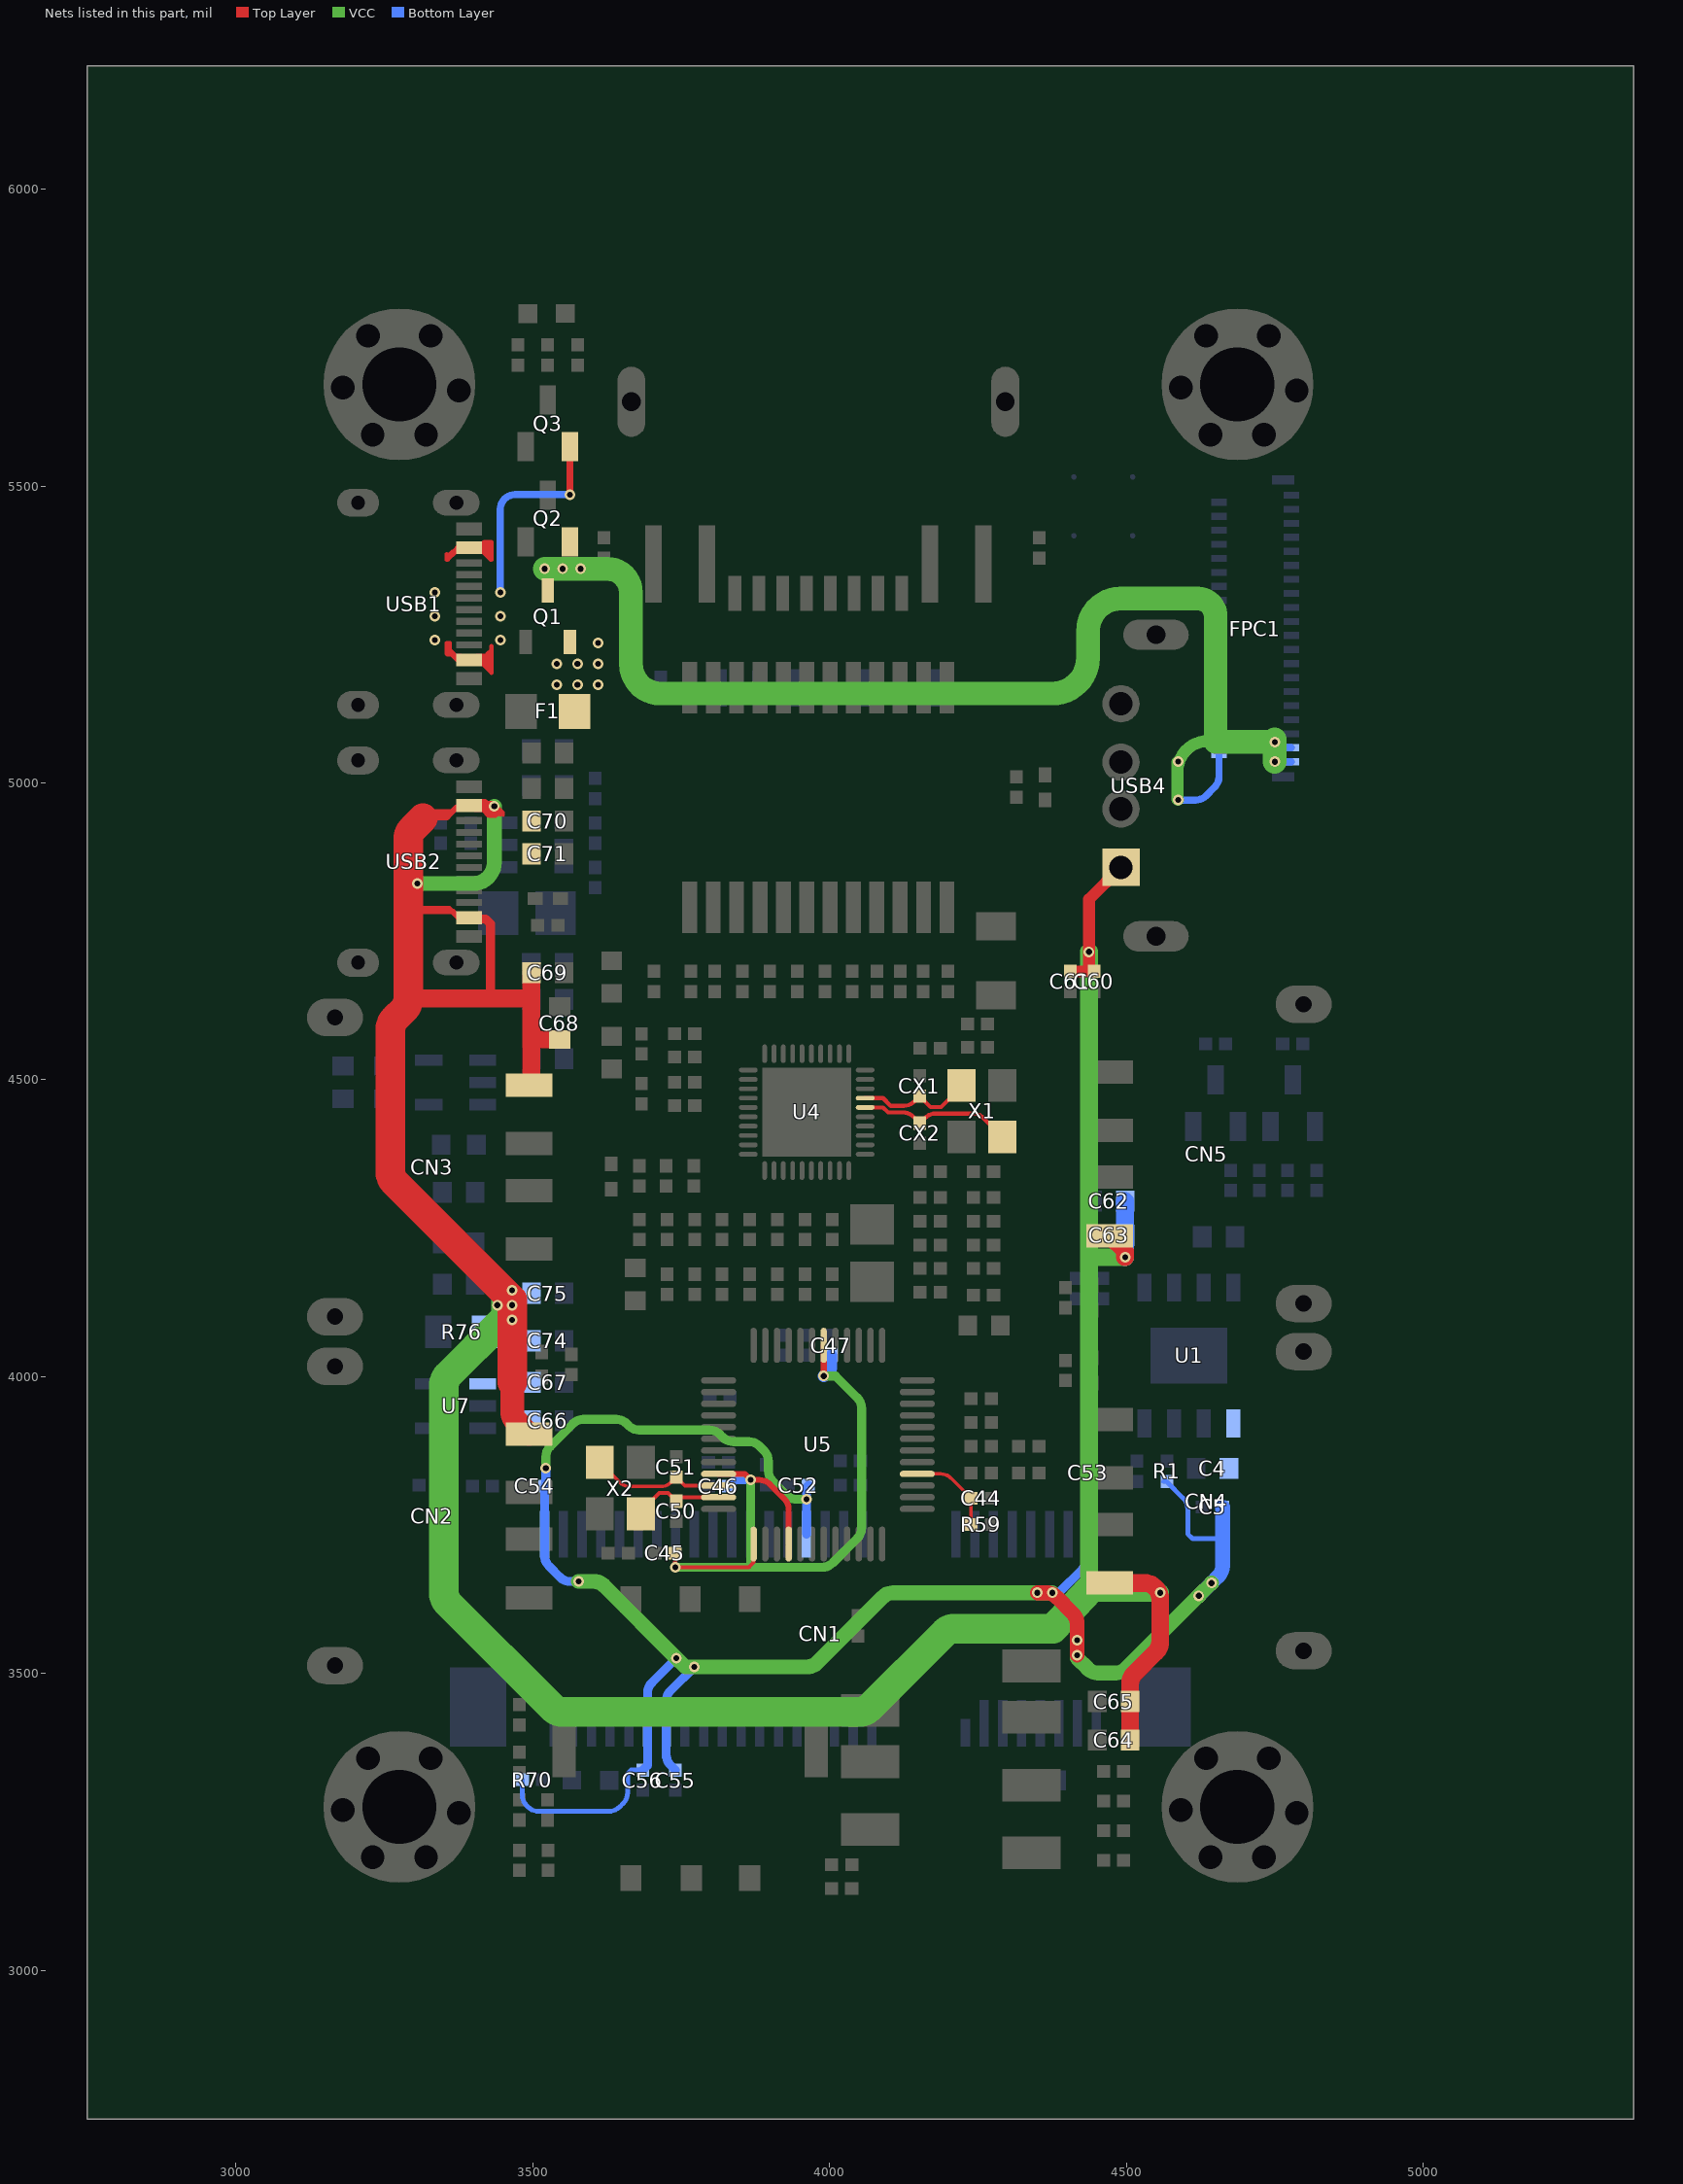
[diagram p0: the nets of this part, all layers, seen from the top]
# Altium PCB MISC84334.PcbDoc (part 8 of 8)
Units mil, origin at the board's own origin, x right, y up, seen from the top; angles counter-clockwise.
Board outline 2605.13 x 3457.4 mil, 4 copper layers (Top Layer, GND, VCC, Bottom Layer), stack 62.447 mil thick; 209 components, 149 nets, 735 pads, 529 vias.

## Via types
v1: diameter 18, hole 10, Top Layer to Bottom Layer, 529 vias

## Nets (pads, with @x,y where several pads share a name; then routed paths per layer and width w, separated by ;. In a path a pad name is that pad's centre, name@x,y a point inside that pad or via, vN(x,y) a via of type N, cw(c..) or ccw(c..) an arc to the next point about the centre after c; other vN are vias at no path point) (continued)
VCC5V0_SYS: FPC1.1 FPC1.2 FPC1.3 FPC1.4 Q1.3 Q2.2 | length 2196
  VCC w20: v1(4587.29,4971.19) 4586.29,4972.19 4586.29,5019.08 ; v1(4587.29,5036.19) 4586.29,5035.19 4586.29,5019.08 ; 4640.59,5070.59 4637.8,5070.59 ccw(c4637.8,5019.08) 4589.01,5035.61 ccw(c4637.8,5019.08) 4586.29,5019.08
  VCC w40: v1(3520.59,5360.59) v1(3550.59,5360.59) v1(3580.59,5360.59) 3625.59,5360.59 cw(c3625.59,5320.59) 3665.59,5320.59 3665.59,5200.59 ccw(c3715.59,5200.59) 3715.59,5150.59 4375.59,5150.59 ccw(c4375.59,5210.59) 4435.59,5210.59 4435.59,5255.59 cw(c4490.59,5255.59) 4490.59,5310.59 4620.59,5310.59 cw(c4620.59,5280.59) 4650.59,5280.59 4650.59,5069.06 v1(4750.2,5069.06) ; v1(4750.29,5035.68) 4750.29,5069.06 v1@4750.29,5073.19
  Bottom Layer w12: v1(4587.29,4971.19) 4616.94,4971.19 ccw(c4616.94,4996.19) 4634.61,4978.51 4648.95,4992.85 ccw(c4631.27,5010.53) 4656.27,5010.53 FPC1.2@4656.27,5047.49 ; v1(4587.29,5036.19) 4614.89,5063.79 cw(c4632.57,5046.11) 4632.57,5071.11 FPC1.4@4656.27,5071.11 ; v1(4750.2,5069.06) 4759.95,5059.3 FPC1.3@4778.31,5059.3 ; v1(4750.29,5035.68) FPC1.1@4778.31,5035.68
VCC5V0_USB_HOST: C60.2 C61.2 C62.2 C63.2 C64.2 C65.2 C66.2 C67.2 C68.2 C69.2 C70.2 C71.2 C74.2 C75.2 CN2.1 CN3.1 CN4.1 CN5.1 R76.2 U7.1 USB2.2 USB2.11 USB4.1 | length 6504.3
  Top Layer w5: 3310.59,4781.94 3363.71,4781.94 USB2.11@3374.22,4771.43 ; 3313.18,4785.39 3313.32,4785.53 3365.65,4785.53 ; 3313.47,4787.58 3357.58,4787.58 3360.59,4790.59 ; 3315.59,4790.59 3360.59,4790.59 ; USB2.11@3388.24,4777.74 3374.8,4777.74 3367.01,4785.53 3365.65,4785.53 ; USB2.2@3402.68,4953.54 3415.71,4953.54 3426.01,4943.23 3437.26,4943.23 3437.72,4943.7 ; USB2.2@3408.37,4965.07 3415.8,4965.07 ; USB2.2@3410.86,4970.27 3420.68,4970.27 3428.42,4962.53 v1@3437.53,4962.53 ; USB2.2@3412.04,4966.85 3419.47,4966.85 3427.01,4959.32 3439.46,4959.32 3445.59,4953.18 3445.59,4945.59 ; 3414.96,4954.56 3414.96,4959.32 ; 3425.84,4967.44 3433.93,4967.44 v1@3438.83,4962.53 ; v1(3435.59,4960.59) v1@3437.53,4962.53 ; 3437.77,4947.77 3426.51,4947.77 3423.04,4951.24 ; 3438.76,4951.24 3423.04,4951.24 ; 3440.59,4945.59 3440.59,4953.67 3438.81,4955.45 3425.42,4955.45 3415.8,4965.07 ; 3450.59,4945.59 3450.59,4950.77 v1@3438.83,4962.53 ; 3360.59,4790.59 3365.65,4785.53 ; 3414.96,4959.32 3423.04,4951.24 ; 3414.96,4959.32 3414.96,4964.23 3415.8,4965.07 ; v1@3437.53,4962.53 v1@3438.83,4962.53
  Top Layer w7: 3331.16,4950.71 3332.7,4952.25 3362.98,4952.25 3371.57,4960.84 3391.86,4960.84 USB2.2@3393.1,4962.08 ; 3333.25,4944.35 3352.35,4944.35 3356.11,4940.59 ; 3334.31,4948.02 3361.5,4948.02 3362.52,4947 ; 3335.59,4940.59 3356.11,4940.59 ; USB2.2@3385.82,4955.77 3371.29,4955.77 3362.52,4947 ; 3356.11,4940.59 3362.52,4947
  Top Layer w15: USB2.11@3391.15,4771.09 3420.52,4771.09 3428.97,4762.64 3428.97,4639.72 3429.51,4639.18
  Top Layer w20: C61.2@4405.59,4682.63 4432.75,4682.63 ; C60.2@4445.59,4682.63 4432.75,4682.63 ; USB4.1@4491.06,4857.8 4437.29,4804.03 v1(4437.29,4715.59) 4437.29,4687.17 4432.75,4682.63
  Top Layer w30: 3300.59,4630.59 3307.01,4637.01 3498.03,4637.01 ; CN3.1@3493.98,4490.89 3498.03,4494.94 3498.03,4567.79 ; C69.2@3498.03,4680.59 3498.03,4637.01 ; 3498.27,4568.03 3498.03,4567.79 ; 3505.59,4568.03 C68.2@3545.59,4568.03 ; CN4.1@4472.2,3652.58 4530.55,3652.58 cw(c4530.55,3627.58) 4548.22,3645.26 4549.97,3643.51 cw(c4532.29,3625.84) 4555.39,3635.4 cw(c4532.29,3625.84) 4557.29,3625.84 4557.29,3554.05 cw(c4532.29,3554.05) 4549.97,3536.37 4513.84,3500.24 ccw(c4531.52,3482.56) 4506.52,3482.56 C65.2@4506.52,3453.09 C64.2@4506.52,3388.09 ; CN5.1@4472.2,4237.58 4498.15,4211.63 v1(4498.15,4201.19) ; 3498.03,4567.79 3498.03,4637.01
  Top Layer w40: 3465.59,3990.59 3465.59,3942.14 ccw(c3490.59,3942.14) 3472.91,3924.46 CN2.1@3493.98,3903.39
  Top Layer w50: 3315.59,4940.59 3297.91,4922.91 ccw(c3315.59,4905.24) 3290.59,4905.24 3290.59,4635.95 cw(c3265.59,4635.95) 3283.27,4618.27 3267.91,4602.91 ccw(c3285.59,4585.24) 3260.59,4585.24 3260.59,4344.95 ccw(c3285.59,4344.95) 3267.91,4327.27 3465.59,4129.59 v1(3465.59,4120.59) v1(3465.59,4095.59) 3465.59,3990.59
  VCC w25: v1(3305.59,4830.59) 3399.78,4830.59 ccw(c3399.78,4866.4) 3435.59,4866.4 v1(3435.59,4960.59)
  VCC w30: v1(4437.29,4715.59) 4437.29,4199.3 ; v1(4498.15,4201.19) 4439.18,4201.19 4437.29,4199.3 ; v1(4557.29,3636.19) 4456.86,3636.19 ; 4437.29,3655.76 4437.29,3640.92 4437.29,3631.19 4442.29,3636.19 4456.86,3636.19 ; 4437.29,3655.76 4437.29,4199.3 ; 4437.29,3655.76 4456.86,3636.19
  VCC w50: 3455.59,4135.59 3455.59,4110.95 cw(c3430.59,4110.95) 3453.48,4100.9 cw(c3430.59,4110.95) 3448.27,4093.27 3357.91,4002.91 ccw(c3375.59,3985.24) 3350.59,3985.24 3350.59,3635.95 ccw(c3375.59,3635.95) 3357.91,3618.27 3533.27,3442.91 ccw(c3550.95,3460.59) 3550.95,3435.59 4050.24,3435.59 ccw(c4050.24,3460.59) 4067.91,3442.91 4193.27,3568.27 cw(c4210.95,3550.59) 4210.95,3575.59 4376.54,3575.59 4378.16,3577.21 ccw(c4360.48,3594.88) 4378.81,3577.88 4437.29,3640.92
  Bottom Layer w30: v1(4498.15,4201.19) C63.2@4498.15,4238.09 C62.2@4498.15,4295.59
  other v1: 3440.59,4120.59 3465.59,4145.59
VCC5V0_USB_VBUS: F1.1 Q1.2 Q3.2 USB1.2 USB1.11 | length 891.9
  Top Layer w7: 3355.59,5385.59 3355.59,5380.59 ; 3359.37,5221.75 3359.37,5219.4 3356.45,5216.48 ; USB1.2@3373.17,5395.16 3370.55,5392.54 3370.55,5389.77 ; USB1.11@3373.2,5206.78 3363.49,5216.48 3356.45,5216.48 ; USB1.2@3375.95,5399.08 3366.64,5389.77 ; USB1.2@3376.74,5389.28 3370.55,5389.28 ; USB1.11@3378.12,5214.41 3370.34,5214.41 3360.59,5224.16 3360.59,5235.59 3355.59,5235.59 3355.59,5217.34 3356.45,5216.48 ; USB1.11@3393.1,5207.1 3409.09,5207.1 3430.59,5185.59 3430.59,5223.59 ; USB1.2@3401.43,5391.03 3413.85,5391.03 3429.29,5375.59 3430.59,5375.59 3430.59,5405.59 ; USB1.11@3406.81,5214.49 3414.83,5214.49 ; USB1.11@3414.18,5203.92 3414.83,5204.56 3414.83,5214.49 ; 3417.14,5390.24 3418.19,5391.29 3418.19,5405.59 ; 3418,5202.33 3418,5211 3421.49,5214.49 ; 3421.4,5388.01 3421.4,5402.38 3418.19,5405.59 ; 3421.78,5197.22 3421.78,5214.2 3421.49,5214.49 ; 3425.92,5193.17 3425.92,5217.22 3425.07,5218.07 ; 3426.1,5381.16 3426.1,5401.1 3430.59,5405.59 ; 3430.59,5230.59 3430.59,5223.59 ; 3355.59,5380.59 3364.77,5389.77 3366.64,5389.77 ; 3355.59,5380.59 3355.59,5375.59 3356.86,5375.59 3370.55,5389.28 ; 3366.64,5389.77 3370.55,5389.77 ; 3370.55,5389.28 3370.55,5389.77 ; 3370.55,5389.77 3386.79,5389.77 USB1.2@3393.1,5396.08 3408.68,5396.08 3418.19,5405.59 ; 3414.83,5214.49 3421.49,5214.49 ; 3418.19,5405.59 3430.59,5405.59 ; 3421.49,5214.49 3425.07,5218.07 ; 3425.07,5218.07 3430.59,5223.59
  Top Layer w12: v1(3562.99,5485.59) Q3.2@3562.99,5566.22
  Bottom Layer w12: v1(3445.59,5320.59) 3445.59,5460.59 cw(c3470.59,5460.59) 3470.59,5485.59 v1(3562.99,5485.59)
  other v1: 3540.59,5165.59 3575.59,5165.59 3610.59,5165.59 3540.59,5200.59 3575.59,5200.59 3610.59,5200.59 3610.59,5235.59 3335.59,5240.59 3445.59,5240.59 3335.59,5280.59 3445.59,5280.59 3335.59,5320.59
VCC_1V8_USB: C45.2 C46.2 C47.2 U5.6 U5.21 U5.25 U5.28 | length 1314.8
  Top Layer w7: C45.2@3740.18,3703.09 v1(3740.18,3679.19) 3864.29,3679.19 3872.32,3687.22 U5.25@3872.32,3718.27
  Top Layer w10: U5.21@3813.27,3836.38 3857.1,3836.38 v1(3867.29,3826.19) 3881.94,3826.19 cw(c3881.94,3801.19) 3899.61,3818.87 3924.06,3794.42 cw(c3906.38,3776.75) 3931.38,3776.75 U5.28@3931.38,3718.27 ; v1(3990.43,4001.19) U5.6@3990.43,4052.91
  VCC w15: v1(3740.18,3679.19) 3868.74,3679.19 ; v1(3867.29,3826.19) 3867.29,3680.64 3868.74,3679.19 ; v1(3990.43,4001.19) 4010.29,4001.19 4046.97,3964.51 cw(c4029.29,3946.84) 4054.29,3946.84 4054.29,3745.55 cw(c4029.29,3745.55) 4046.97,3727.87 4005.61,3686.51 cw(c3987.94,3704.19) 3987.94,3679.19 3868.74,3679.19
  Bottom Layer w15: C46.2@3830.13,3815.59 3840.73,3826.19 v1(3867.29,3826.19)
  Bottom Layer w20: v1(3990.43,4001.19) 4003.09,4013.85 C47.2@4003.09,4036.05
VCC_4G: C4.2 C5.2 C52.2 C53.2 C54.2 C55.2 C56.2 CN1.2 CN1.24 CN1.39 CN1.41 CN1.52 R1.2 R70.2 U1.1 | length 3494.3
  Top Layer w25: v1(4350.38,3636.19) 4364.94,3636.19 cw(c4364.94,3611.19) 4374.5,3634.29 cw(c4364.94,3611.19) 4382.61,3628.87 4409.97,3601.51 cw(c4392.29,3583.84) 4417.29,3583.84 v1(4417.29,3556.19) v1(4417.29,3531.19)
  VCC w15: v1(3522.29,3846.19) 3522.29,3864.84 cw(c3547.29,3864.84) 3529.61,3882.51 3567.97,3920.87 cw(c3585.65,3903.19) 3585.65,3928.19 3640.94,3928.19 cw(c3640.94,3903.19) 3658.61,3920.87 3661.97,3917.51 ccw(c3679.65,3935.19) 3679.65,3910.19 3797.94,3910.19 cw(c3797.94,3885.19) 3815.61,3902.87 3820.47,3898.01 ccw(c3838.15,3915.69) 3838.15,3890.69 3864.34,3890.69 cw(c3864.34,3865.69) 3882.02,3883.37 3889.97,3875.42 cw(c3872.29,3857.74) 3897.29,3857.74 3897.29,3841.55 ccw(c3922.29,3841.55) 3904.61,3823.87 3927.72,3800.76 ccw(c3945.4,3818.44) 3945.4,3793.44 v1(3961.34,3793.44)
  VCC w25: v1(3577.29,3655.19) 3602.94,3655.19 cw(c3602.94,3630.19) 3620.61,3647.87 v1(3742.29,3526.19) 3757.29,3511.19 v1(3772.29,3511.19) 3961.94,3511.19 ccw(c3961.94,3536.19) 3979.61,3518.51 4089.97,3628.87 cw(c4107.65,3611.19) 4107.65,3636.19 v1(4350.38,3636.19) v1(4375.29,3636.19) ; v1@4417.29,3526.19 4434.97,3508.51 ccw(c4452.65,3526.19) 4452.65,3501.19 4481.94,3501.19 ccw(c4481.94,3526.19) 4499.61,3508.51 v1(4622.29,3631.19) v1(4643.62,3652.52) ; v1(4417.29,3531.19) v1(4417.29,3556.19)
  Bottom Layer w8: R70.2@3482.66,3321.19 3482.66,3295.34 ccw(c3507.66,3295.34) 3489.99,3277.67 3492.14,3275.51 ccw(c3509.82,3293.19) 3509.82,3268.19 3628.94,3268.19 ccw(c3628.94,3293.19) 3646.61,3275.51 3652.68,3281.58 ccw(c3635,3299.26) 3660,3299.26 3660,3331.97 3665.66,3337.63 C56.2@3685.59,3337.63 ; R1.2@4562.63,3823.55 4567.93,3823.55 4596.36,3795.12 cw(c4578.68,3777.44) 4603.68,3777.44 4603.68,3735.45 4611.68,3727.45 4662.33,3727.45
  Bottom Layer w15: v1(3522.29,3846.19) 3522.29,3817.81 C54.2@3520.51,3816.03 3520.39,3815.91 CN1.52@3520.39,3735.04 3520.39,3698.52 ccw(c3545.39,3698.52) 3527.71,3680.85 3546.04,3662.51 ccw(c3563.72,3680.19) 3563.72,3655.19 v1(3577.29,3655.19) ; C56.2@3685.59,3337.63 3693.62,3345.66 CN1.41@3693.62,3416.14 3693.62,3467.16 cw(c3718.62,3467.16) 3700.94,3484.84 v1(3742.29,3526.19) ; C55.2@3740.59,3337.63 3732.44,3345.78 cw(c3750.12,3363.46) 3725.12,3363.46 CN1.39@3725.12,3416.14 3725.12,3453.66 cw(c3750.12,3453.66) 3732.44,3471.34 v1(3772.29,3511.19) ; CN1.24@3961.34,3735.04 v1(3961.34,3793.44) 3961.34,3813.78 C52.2@3964.59,3817.03 ; v1(4375.29,3636.19) 4386.29,3636.19 4426.45,3676.35 ccw(c4408.78,3694.03) 4433.78,3694.03 CN1.2@4433.78,3735.04 4433.78,3818.79 C53.2@4436.02,3821.03
  Bottom Layer w25: v1(4622.29,3631.19) v1(4643.62,3652.52) 4655,3663.9 ccw(c4637.33,3681.58) 4662.33,3681.58 4662.33,3727.45 C5.2@4662.33,3780.59
XIN: C51.1 U5.22 X2.3 | length 227.2
  Top Layer w6: X2.3@3613.28,3855.76 3646.53,3822.51 ccw(c3664.2,3840.19) 3664.2,3815.19 3715.8,3815.19 ccw(c3715.8,3840.19) 3733.48,3822.51 C51.1@3742.02,3831.05 3756.38,3816.69 U5.22@3813.27,3816.69
XOUT: C50.2 U5.23 X2.1 | length 156.3
  Top Layer w6: X2.1@3682.18,3769.14 3682.18,3773.08 3713.29,3804.19 3728.26,3804.19 C50.2@3742.02,3790.43 3748.6,3797.01 U5.23@3813.27,3797.01
XRSTJ: C44.2 R59.1 U5.40 | length 149.8
  Top Layer w6: U5.40@4147.91,3836.38 4187.42,3836.38 cw(c4187.42,3811.38) 4205.09,3829.06 4231.24,3802.91 cw(c4213.56,3785.24) 4238.56,3785.24 R59.1@4238.56,3751.19
XTAL_IN: CX2.2 U4.36 X1.3 | length 262
  Top Layer w7: U4.36@4060.16,4453.49 4090.43,4453.49 4098.78,4445.14 4123.98,4445.14 cw(c4123.98,4420.14) 4141.66,4437.82 CX2.2@4152.35,4427.13 4161.09,4435.87 cw(c4178.77,4418.19) 4178.77,4443.19 4241.78,4443.19 cw(c4241.78,4418.19) 4259.45,4435.87 X1.3@4291.54,4403.78
XTAL_OUT: CX1.2 U4.37 X1.1 | length 197.3
  Top Layer w7: U4.37@4060.16,4469.19 4090.29,4469.19 4103.29,4456.19 4125.33,4456.19 ccw(c4125.33,4481.19) 4143.01,4463.51 CX1.2@4152.05,4472.55 4170.41,4454.19 4188.29,4454.19 4222.64,4488.54 X1.1@4222.64,4490.4
pads on no net: AUDIO1.7 AUDIO1.8 CARD1.C6 CN1.1 CN1.3 CN1.5 CN1.6 CN1.7 CN1.13 CN1.16 CN1.17 CN1.19 CN1.20 CN1.22 CN1.25 CN1.28 CN1.30 CN1.32 CN1.33 CN1.44 CN1.45 CN1.46 CN1.47 CN1.48 CN1.49 CN1.51 FPC1.26 FPC1.27 FPC1.29 FPC1.30 U1.4 U1.6 U1.7 U3.4 U5.2 U5.44 U5.46 USB1.3 USB1.4 USB1.5 USB1.6 USB1.7 USB1.8 USB1.9 USB1.10 USB2.3 USB2.4 USB2.9 USB2.10

## Polygon pours and split planes (outlines as drawn)
VCC5V0_USB_VBUS on Top Layer (solid, remove dead copper, pour order 6): 3530.81,5260.59 3524.86,5254.64 3524.86,5219.86 3518.39,5213.39 3474.6,5213.39 3465.59,5222.4 3465.59,5395.59 3450.59,5410.59 3325.59,5410.59 3305.59,5390.59 3305.59,5211.48 3326.6,5190.47 3416.98,5190.47 3452.5,5154.94 3534.14,5154.94 3540.83,5148.26 3540.83,5082.82 3548.06,5075.59 3609.55,5075.59 3620.59,5086.63 3620.59,5245.59 3605.59,5260.59
IN_5V on Bottom Layer (solid, remove dead copper, pour order 16): 4660.85,4259.43 4655.29,4253.86 4655.29,4134.28 4666.85,4122.71 4722.71,4122.71 4730.59,4130.59 4730.59,4251.97 4723.14,4259.43
VCC_4G on Bottom Layer (solid, remove dead copper, pour order 18): 4659.85,3949.85 4649.42,3939.42 4649.42,3763.91 4657.74,3755.59 4705.33,3755.59 4715.59,3765.86 4715.59,3941.13 4706.87,3949.85
VCC5V0_SYS on Top Layer (solid, remove dead copper, pour order 8): 3583.41,5439.8 3534.96,5439.8 3524.86,5429.71 3524.86,5379.86 3490.59,5345.59 3490.59,5295.59 3505.59,5280.59 3580.59,5280.59 3590.59,5290.59 3590.59,5432.62
IN_5V on Top Layer (solid, remove dead copper, pour order 10): 3529.83,5137.47 3529.83,4979.01 3522.71,4971.88 3429.3,4971.88 3422.23,4978.95 3422.23,5141.89 3432.9,5152.56 3514.74,5152.56
VCC5V0_USB_VBUS on Bottom Layer (solid, remove dead copper, pour order 20): 3320.2,5350.59 3305.59,5335.98 3305.59,5200.59 3340.59,5165.59 3410.59,5165.59 3425.59,5150.59 3615.59,5150.59 3625.59,5160.59 3625.59,5330.59 3605.59,5350.59
IN_5V on Bottom Layer (solid, remove dead copper, pour order 22): 3427.77,5084.02 3420.59,5076.84 3420.59,4977.3 3431.66,4966.23 3459.95,4966.23 3480.59,4945.59 3480.59,4880.59 3485.59,4875.59 3570.59,4875.59 3575.59,4880.59 3575.59,4910.59 3570.59,4915.59 3535.59,4915.59 3531.58,4919.6 3531.58,5078.86 3526.42,5084.02
$5N2260 on Bottom Layer (solid, remove dead copper, pour order 24): 3570.99,4873.47 3503.47,4873.47 3490.59,4860.59 3490.59,4750.59 3505.59,4735.59 3570.59,4735.59 3580.59,4745.59 3580.59,4863.87
VCC3V3_SYS on Bottom Layer (solid, remove dead copper, pour order 26): 3475.59,4830.59 3380.59,4830.59 3360.59,4810.59 3360.59,4760.59 3415.59,4705.59 3415.59,4665.59 3385.59,4635.59 3385.59,4522.52 3394.4,4513.71 3518.38,4513.71 3525.59,4520.92 3525.59,4713.21 3490.59,4748.21 3490.59,4815.59
VCC1V8 on Bottom Layer (solid, remove dead copper, pour order 28): 3357.5,4600.59 3240.59,4600.59 3200.59,4560.59 3125.59,4560.59 3115.59,4550.59 3115.59,4503.69 3115.78,4503.5 3353.58,4503.5 3368.2,4518.12 3368.2,4589.89
GND on Bottom Layer (solid, remove dead copper, pour order 30): 3384.93,4410.59 3140.59,4410.59 3115.59,4435.59 3115.59,4480.59 3135.59,4500.59 3355.59,4500.59 3365.59,4510.59 3516.34,4510.59 3525.59,4519.84 3525.59,4715.59 3540.59,4730.59 3570.59,4730.59 3585.59,4745.59 3585.59,4775.59 3620.59,4810.59 3620.59,4985.59 3615.59,4990.59 3595.59,4990.59 3575.59,4970.59 3535.59,4970.59 3530.59,4975.59 3530.59,5080.59 3525.59,5085.59 3425.59,5085.59 3420.59,5080.59 3420.59,5030.59 3395.59,5005.59 3320.59,5005.59 3300.59,5025.59 3300.59,5135.59 3330.59,5165.59 3410.59,5165.59 3425.59,5150.59 3640.59,5150.59 3660.59,5130.59 3660.59,4541.2 3579.67,4460.27 3579.67,3904.67 3570.59,3895.59 3539.84,3895.59 3525.59,3909.84 3525.59,4165.59 3505.59,4185.59 3480.59,4185.59 3422.76,4127.76 3387.67,4127.76 3375.59,4139.84 3375.59,4326.06 3385.31,4335.79 3438.79,4335.79 3445.59,4342.59 3445.59,4470.59 3440.59,4475.59 3392.73,4475.59 3388.72,4471.58 3388.72,4414.38
IN_5V on Bottom Layer (solid, remove dead copper, pour order 32): 3359.72,4272.96 3240.36,4272.96 3225.59,4258.19 3225.59,3980.59 3250.59,3955.59 3363.78,3955.59 3374.95,3966.76 3374.95,4257.74
VCC5V0_USB_HOST on Bottom Layer (solid, remove dead copper, pour order 34): 3475.59,4170.59 3425.59,4120.59 3395.59,4120.59 3385.59,4110.59 3385.59,3978 3394.4,3969.18 3450.64,3969.18 3462.37,3957.45 3462.37,3908.81 3475.59,3895.59 3517.6,3895.59 3525.59,3903.58 3525.59,4160.59 3515.59,4170.59
GND on Top Layer (solid, remove dead copper, pour order 14): 3000,5952.76 3000,3000 4968.5,3000 4968.5,5952.76
GND on Bottom Layer (solid, remove dead copper, pour order 36): 3000,5952.76 3000,3000 4968.5,3000 4968.5,5952.76
GND on GND (solid, remove dead copper): 3000,5952.76 3000,3000 4968.5,3000 4968.5,5952.76
GND on VCC (solid, remove dead copper): 3000,5952.76 3000,3000 4968.5,3000 4968.5,5952.76
LDO_OUT on Top Layer (solid, remove dead copper, pour order 0): 4080.91,4324.82 4040.29,4324.82 4032.66,4317.19 4032.66,4220.82 4035.29,4218.19 4106.29,4218.19 4111.29,4223.19 4111.29,4294.44
1V05_PHY on Top Layer (solid, remove dead copper, pour order 2): 4037.24,4202.46 4029.58,4194.81 4029.58,4123.9 4037.29,4116.19 4156.77,4116.19 4164.85,4124.27 4164.85,4194.23 4156.62,4202.46
VCC5V0_USB_HOST on Top Layer (solid, remove dead copper, pour order 12): 3503.81,4964.6 3437.99,4964.6 3425.09,4951.7 3425.09,4917.56 3481.31,4861.34 3518.8,4861.34 3524.82,4867.36 3524.82,4943.59
IN_5V on VCC (solid, remove dead copper): 3580.59,5075.59 3435.59,5075.59 3425.59,5065.59 3425.59,5000.59 3460.59,4965.59 3460.59,4560.59 3225.59,4325.59 3225.59,4187.56 3237.56,4175.59 3400.59,4175.59 3600.59,4375.59 3600.59,5055.59
VCC3V3_USB on Top Layer (solid, remove dead copper, pour order 4): 4219.82,3973.72 4192.29,3946.19 4192.29,3876.19 4197.29,3871.19 4247.29,3871.19 4252.29,3876.19 4252.29,3971.58 4250.15,3973.72

## Keep-outs
Top Layer:
  region: 3682.23,5117.32 3682.23,4833.86 4280.65,4833.86 4280.65,5117.32
  region: 3800.88,3816.69 3773.3,3816.69 3773.3,3839.88 3748.04,3865.13 3742.02,3865.13 3703.96,3903.19 3590.29,3903.19 3577.29,3890.19 3577.29,3738.18 3587.29,3728.18 3713.85,3728.18 3742.02,3756.35 3745.45,3756.35 3766.42,3777.32 3800.41,3777.32 3800.88,3777.79
  region: 4337.29,4511.19 4318.29,4530.19 4172.32,4530.19 4119.29,4477.16 4119.29,4424.19 4150.43,4393.05 4152.35,4393.05 4201.31,4344.09 4310.14,4344.09 4337.29,4371.24
VCC:
  region: 3643.74,3374.83 3643.74,3334.27 3670.59,3334.27 3670.59,3374.83
  region: 3682.23,5117.32 3682.23,4833.86 4280.65,4833.86 4280.65,5117.32
  region: 3682.23,5117.32 3682.23,4833.86 4280.65,4833.86 4280.65,5117.32
Bottom Layer:
  region: 3682.23,5117.32 3682.23,4833.86 4280.65,4833.86 4280.65,5117.32
Board Outline Layer:
  lines w10: 3706.44,5845.59 3245.59,5846.2 ccw(c3245.59,5696.2) 3095.59,5696.2 3095.59,3240.59 ccw(c3245.59,3240.59) 3245.59,3090.59 4717.24,3090.59 ccw(c4717.24,3240.59) 4867.24,3240.59 4867.24,5696.2 ccw(c4717.24,5696.2) 4717.24,5846.2 ; 4301.44,5846.09 4717.24,5846.09

## Silkscreen, mask and mechanical layers (free items; w line width, h text height)
Top Silkscreen Layer:
  text "POWER" at 3415.59,5395.59 h60 r270
  text "RJ45" at 4052.91,5283.08 h60 r180
  text "USB4" at 4368.4,5061.24 h60 r270
  text "USB3" at 3415.59,4934.49 h60 r270
  text "USB6" at 4368.4,4446.81 h60 r270
  text "USB2" at 3536.53,4419.29 h60 r270
  text "USB5" at 4368.4,3864.22 h60 r270
  text "USB1" at 3530.01,3831.48 h60 r270
  text "SIM" at 3850.52,3718.66 h60 r180
  text "AUDIO" at 4294.83,3687.11 h60 r180
Bottom Silkscreen Layer:
  text "[V1.0.2]" at 3871.05,5436.19 h60 r180
  text "mini PCIE" at 3819.49,3357.61 h80 r180